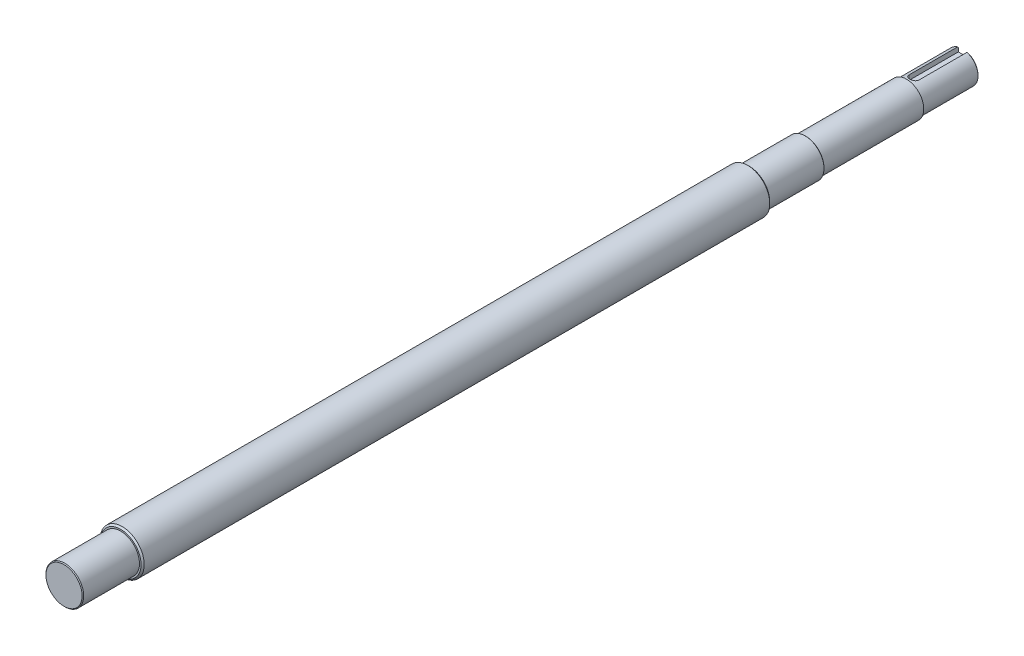
from build123d import *

# Parameters (mm, degrees)
SKETCH1_R           = 12
BOSS_EXTRUDE1_DEPTH = 472
SKETCH2_R           = 11
BOSS_EXTRUDE2_DEPTH = 100
SKETCH4_R           = 14
BOSS_EXTRUDE3_DEPTH = 400
CHAMFER1_SIZE       = 1
CHAMFER2_SIZE       = 0.5
CHAMFER3_SIZE       = 0.5
SKETCH5_R           = 20
SKETCH5_R_2         = 10
CUT_EXTRUDE1_DEPTH  = 36
CUT_EXTRUDE2_DEPTH  = 573.538426658
CHAMFER4_SIZE       = 0.5


with BuildPart() as part:
    # Sketch1 → Boss-Extrude1 (new body)
    with BuildSketch(Plane.XY):
        Circle(SKETCH1_R)
    extrude(amount=-BOSS_EXTRUDE1_DEPTH)

    # Sketch2 → Boss-Extrude2 (add)
    with BuildSketch(Plane(origin=(0, 0, -472), x_dir=(-1, 0, 0), z_dir=(0, 0, -1))):
        Circle(SKETCH2_R)
    extrude(amount=BOSS_EXTRUDE2_DEPTH)

    # Sketch4 → Boss-Extrude3 (add)
    with BuildSketch(Plane.XY.offset(-36)):
        Circle(SKETCH4_R)
    extrude(amount=-BOSS_EXTRUDE3_DEPTH)

    # Chamfer1
    chamfer1_edges = [part.edges().sort_by_distance(p)[0] for p in [
        (-14, 0, -36),
        (-14, 0, -436),
    ]]
    chamfer(chamfer1_edges, length=CHAMFER1_SIZE)

    # Chamfer2
    chamfer2_edges = [part.edges().sort_by_distance(p)[0] for p in [
        (-12, 0, 0),
    ]]
    chamfer(chamfer2_edges, length=CHAMFER2_SIZE)

    # Chamfer3
    chamfer3_edges = [part.edges().sort_by_distance(p)[0] for p in [
        (-12, 0, -472),
    ]]
    chamfer(chamfer3_edges, length=CHAMFER3_SIZE)

    # Sketch5 → Cut-Extrude1 (cut)
    with BuildSketch(Plane(origin=(0, 0, -572), x_dir=(-1, 0, 0), z_dir=(0, 0, -1))):
        Circle(SKETCH5_R)
        Circle(SKETCH5_R_2, mode=Mode.SUBTRACT)
    extrude(amount=-CUT_EXTRUDE1_DEPTH, mode=Mode.SUBTRACT)

    # Sketch6 → Cut-Extrude2 (cut, through all)
    with BuildSketch(Plane(origin=(0, 6.5, 0), x_dir=(1, 0, 0), z_dir=(0, 1, 0))):
        with BuildLine():
            Line((3, 576.648489628), (3, 541))
            ThreePointArc((3, 541), (0, 538), (-3, 541))
            Line((-3, 541), (-3, 576.648489628))
            ThreePointArc((-3, 576.648489628), (0, 579.648489628), (3, 576.648489628))
        make_face()
    extrude(amount=CUT_EXTRUDE2_DEPTH, mode=Mode.SUBTRACT)

    # Chamfer4
    chamfer4_edges = [part.edges().sort_by_distance(p)[0] for p in [
        (5.916079783, -8.062257748, -572),
    ]]
    chamfer(chamfer4_edges, length=CHAMFER4_SIZE)


solid = part.part
